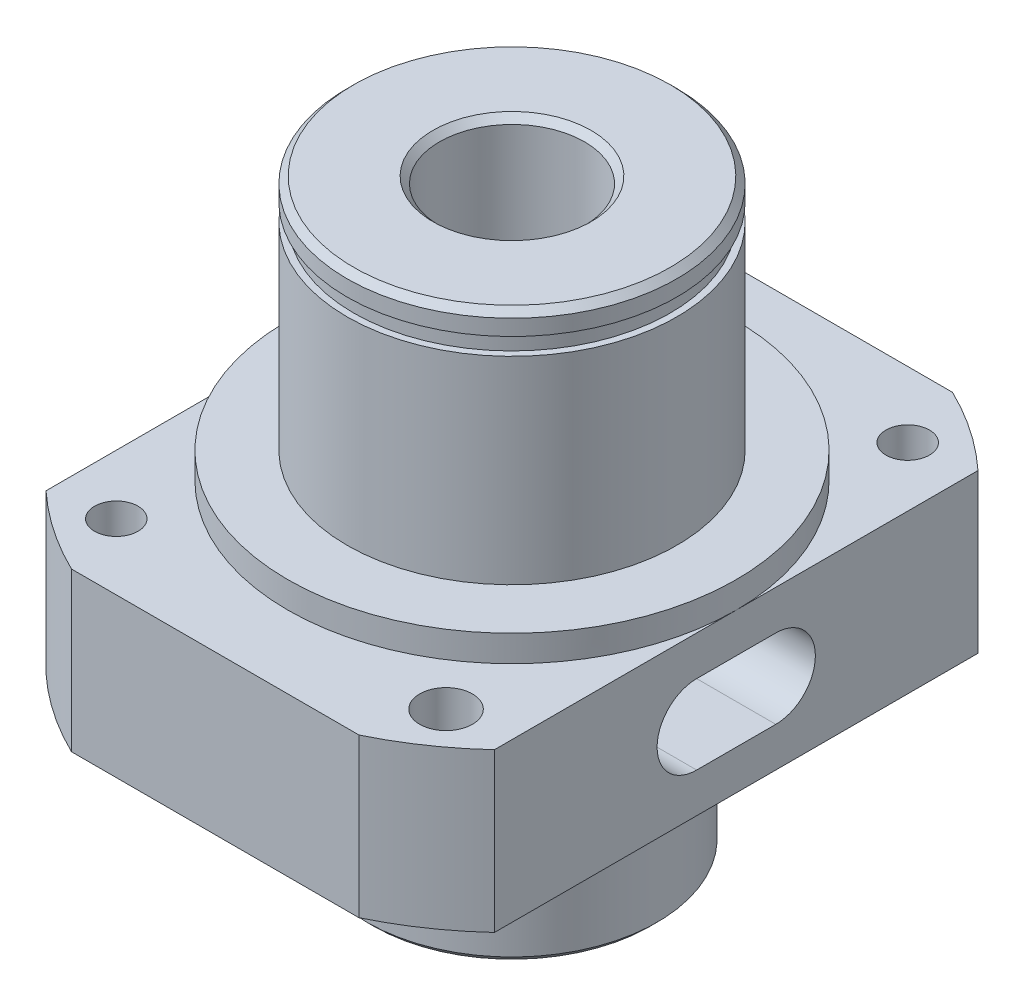
from build123d import *

# Parameters (mm, degrees)
SKETCH2_OUTSIDE_W   = 68.656
SKETCH2_OUTSIDE_H   = 68.656
SKETCH2_OUTSIDE_W_2 = 34
SKETCH2_OUTSIDE_H_2 = 45
CUT_EXTRUDE1_DEPTH  = 43.731721238
SKETCH3_R           = 5.5
CUT_EXTRUDE2_DEPTH  = 53.261362401
M4_TAPPED_HOLE1_D   = 3.3
SKETCH14_R          = 2
CUT_EXTRUDE5_DEPTH  = 38.030392923
CHAMFER1_SIZE       = 0.5
CHAMFER2_SIZE       = 0.5
CUT_EXTRUDE6_DEPTH  = 52.829045911


with BuildPart() as part:
    # Sketch1 → Revolve1 (revolve)
    with BuildSketch(Plane(origin=(0, 0, 0), x_dir=(0, 0, -1), z_dir=(1, 0, 0)), mode=Mode.PRIVATE) as revolve1_sk:
        Polygon((0, -12), (11, -12), (11, 0), (25, 0), (25, 12), (17, 12), (17, 14), (12.5, 14), (12.5, 29), (12, 29), (12, 30.3), (12.5, 30.3), (12.5, 32), (0, 32), align=None)
    revolve(revolve1_sk.sketch.rotate(Axis((0, 78.762169225, 0), (0, -1, 0)), 180), axis=Axis((0, 78.762169225, 0), (0, -1, 0)))

    # Sketch2 outside → Cut-Extrude1 (cut, through all)
    with BuildSketch(Plane(origin=(0, 12, 0), x_dir=(1, 0, 0), z_dir=(0, 1, 0))):
        Rectangle(SKETCH2_OUTSIDE_W, SKETCH2_OUTSIDE_H)
        Rectangle(SKETCH2_OUTSIDE_W_2, SKETCH2_OUTSIDE_H_2, mode=Mode.SUBTRACT)
    extrude(amount=-CUT_EXTRUDE1_DEPTH, mode=Mode.SUBTRACT)

    # Sketch3 → Cut-Extrude2 (cut, through all)
    with BuildSketch(Plane.XZ.offset(12)):
        with Locations(Location((0, 0, 0), (0, 0, 270))):
            Circle(SKETCH3_R)
    extrude(amount=-CUT_EXTRUDE2_DEPTH, mode=Mode.SUBTRACT)

    # M4 Tapped Hole1 (through all)
    with Locations(Plane(origin=(0, 0, 0), x_dir=(-1, 0, 0), z_dir=(0, -1, 0))):
        with Locations((-12.5, 17.5), (12.5, -17.5)):
            Hole(M4_TAPPED_HOLE1_D / 2)

    # Sketch14 → Cut-Extrude5 (cut, through all)
    with BuildSketch(Plane(origin=(0, 12, 0), x_dir=(1, 0, 0), z_dir=(0, 1, 0))):
        with Locations(Location((12.5, -17.5, 0), (0, 0, 270))):
            Circle(SKETCH14_R)
        with Locations(Location((-12.5, 17.5, 0), (0, 0, 270))):
            Circle(SKETCH14_R)
    extrude(amount=-CUT_EXTRUDE5_DEPTH, mode=Mode.SUBTRACT)

    # Chamfer1
    chamfer1_edges = [part.edges().sort_by_distance(p)[0] for p in [
        (0, -12, -11),
        (0, 32, -12.5),
    ]]
    chamfer(chamfer1_edges, length=CHAMFER1_SIZE)

    # Chamfer2
    chamfer2_edges = [part.edges().sort_by_distance(p)[0] for p in [
        (0, 32, 5.5),
        (0, -12, 5.5),
    ]]
    chamfer(chamfer2_edges, length=CHAMFER2_SIZE)

    # Sketch15 → Cut-Extrude6 (cut, through all)
    with BuildSketch(Plane(origin=(17, 0, 0), x_dir=(0, 0, -1), z_dir=(1, 0, 0))):
        with BuildLine():
            Line((-3, 9), (3, 9))
            ThreePointArc((3, 9), (6, 6), (3, 3))
            Line((3, 3), (-3, 3))
            ThreePointArc((-3, 3), (-6, 6), (-3, 9))
        make_face()
    extrude(amount=-CUT_EXTRUDE6_DEPTH, mode=Mode.SUBTRACT)


solid = part.part
